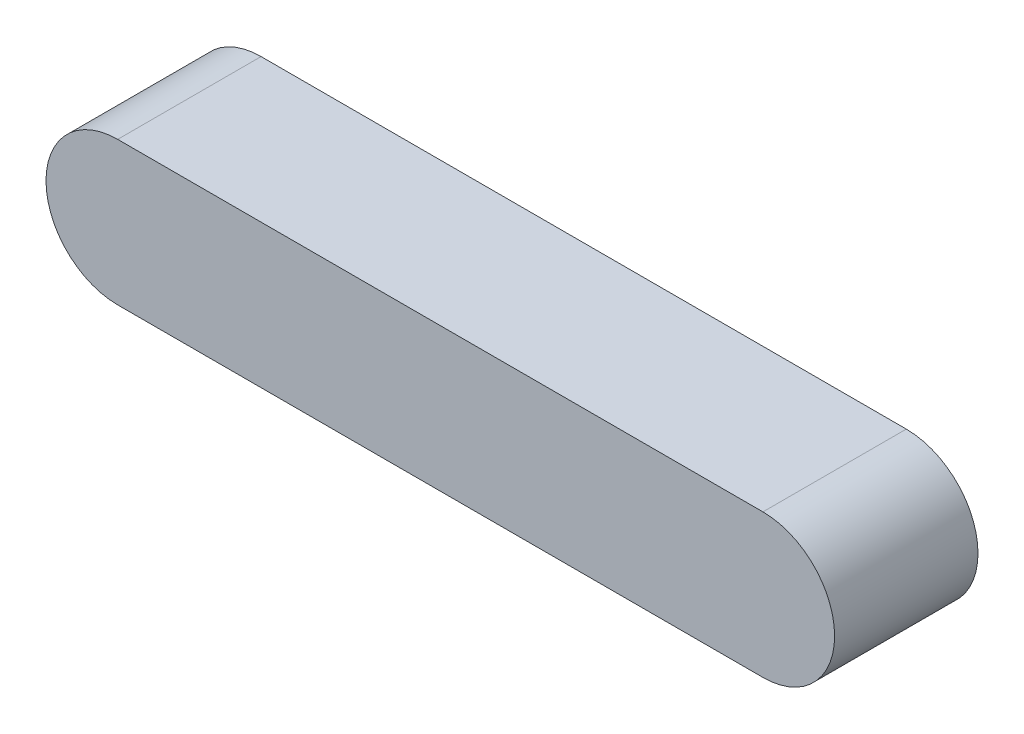
SolidWorks part; units mm, degrees
ref_plane "Front Plane" through (0, 0, 0) normal (0, 0, 1) x (1, 0, 0)
ref_plane "Top Plane" through (0, 0, 0) normal (0, 1, 0) x (1, 0, 0)
ref_plane "Right Plane" through (0, 0, 0) normal (1, 0, 0) x (0, 0, -1)
sketch "Sketch1" plane through (0, 0, 0) normal (0, 0, 1) x (1, 0, 0)
  line L0 (0, 0) -> (18, 0) construction
  line L1 (0, 2) -> (18, 2)
  line L2 (0, -2) -> (18, -2)
  arc A0 (0, 2) -> (0, -2) centre (0, 0) ccw
  arc A1 (18, -2) -> (18, 2) centre (18, 0) ccw
  point P3 (9, 0)
  dimension "D1" = 2
  dimension "D2" = 18
extrude "Boss-Extrude1" add sketch "Sketch1" along normal blind 4
